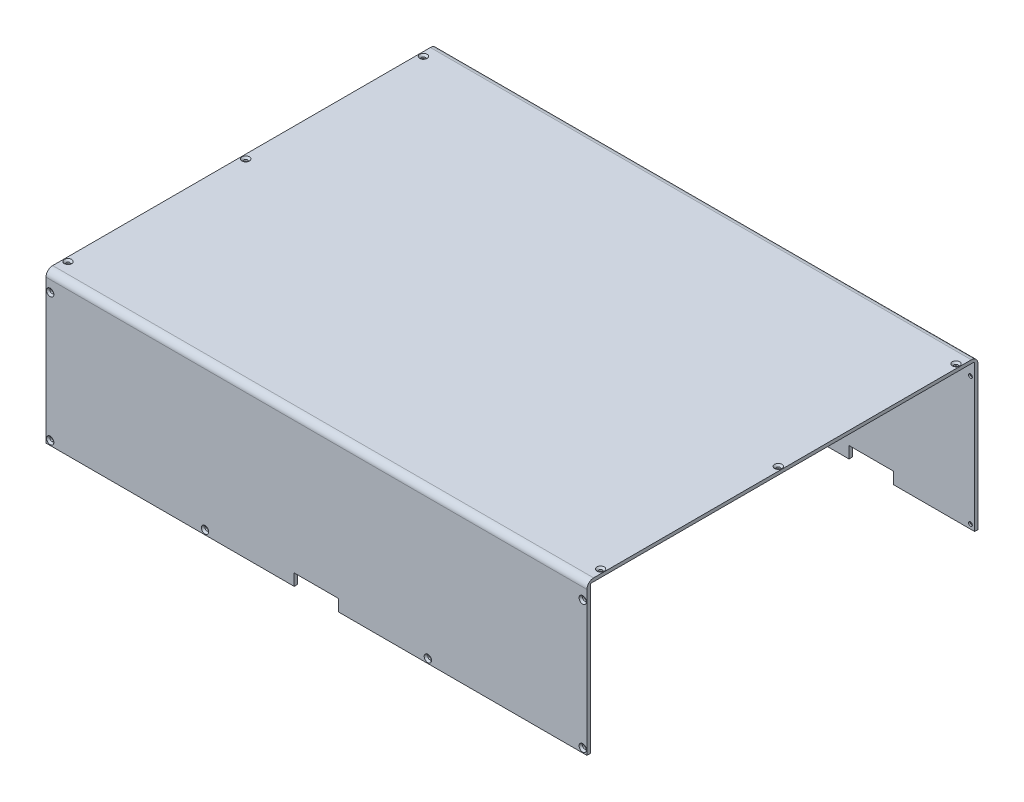
SolidWorks part; units mm, degrees
ref_plane "Front Plane" through (0, 0, 0) normal (0, 0, 1) x (1, 0, 0)
ref_plane "Top Plane" through (0, 0, 0) normal (0, 1, 0) x (1, 0, 0)
ref_plane "Right Plane" through (0, 0, 0) normal (1, 0, 0) x (0, 0, -1)
sketch "Sketch1" plane through (0, 0, 0) normal (0, 0, 1) x (1, 0, 0)
  line L1 (-242.75, 66) -> (242.75, 66)
  line L2 (-242.75, 66) -> (-242.75, -66)
  line L3 (-242.75, -66) -> (242.75, -66)
  line L4 (242.75, 66) -> (242.75, -66)
  line L5 (-242.75, 66) -> (242.75, -66) construction
  line L6 (-242.75, -66) -> (242.75, 66) construction
  point P0 (0, 0)
  dimension "D1" = 132
  dimension "D2" = 485.5
extrude "Boss-Extrude1" add sketch "Sketch1" along normal blind 3
sketch "Sketch2" plane through (0, 66, 0) normal (0, 1, 0) x (1, 0, 0)
  line L0 (-242.75, -3) -> (242.75, -3)
  line L1 (242.75, -3) -> (242.75, 348)
  line L2 (242.75, 348) -> (-242.75, 348)
  line L3 (-242.75, 348) -> (-242.75, -3)
  dimension "D1" = 351
extrude "Boss-Extrude2" add sketch "Sketch2" along normal blind 3
sketch "Sketch3" plane through (0, 66, 0) normal (0, -1, 0) x (1, 0, 0)
  line L0 (242.75, -348) -> (-242.75, -348)
  line L1 (-242.75, -348) -> (-242.75, -345)
  line L2 (-242.75, -348) -> (-242.75, 0) construction
  line L3 (-242.75, -345) -> (242.75, -345)
  line L4 (242.75, 0) -> (242.75, -348) construction
  line L5 (242.75, -345) -> (242.75, -348)
  dimension "D1" = 3
extrude "Boss-Extrude3" add sketch "Sketch3" along normal blind 132
fillet "Fillet1" radius 1 2 edges at (0, 66, -345) (0, 66, 0)
fillet "Fillet2" radius 6 2 edges at (0, 69, -348) (0, 69, 3)
sketch "Sketch4" plane through (0, 0, 3) normal (0, 0, 1) x (1, 0, 0)
  line L6 (20, -55.5) -> (20, -66) construction
  line L7 (-20, -55.5) -> (-20, -66) construction
  line L8 (20, -55.5) -> (20, -66)
  line L9 (-20, -55.5) -> (-20, -66)
  line L10 (-20, -66) -> (20, -66)
  line L11 (-20, -55.5) -> (20, -55.5)
extrude "Cut-Extrude1" cut sketch "Sketch4" against normal blind 4.5
sketch "Sketch5" plane through (0, 0, -348) normal (0, 0, -1) x (-1, 0, 0)
  line L12 (130, -66) -> (170, -66) construction
  line L13 (170, -66) -> (170, -55.5) construction
  line L14 (170, -55.5) -> (130, -55.5) construction
  line L15 (130, -55.5) -> (130, -66) construction
  line L16 (-170, -66) -> (-130, -66) construction
  line L17 (-130, -66) -> (-130, -55.5) construction
  line L18 (-130, -55.5) -> (-170, -55.5) construction
  line L19 (-170, -55.5) -> (-170, -66) construction
  line L20 (130, -66) -> (170, -66)
  line L21 (170, -66) -> (170, -55.5)
  line L22 (170, -55.5) -> (130, -55.5)
  line L23 (130, -55.5) -> (130, -66)
  line L24 (-170, -66) -> (-130, -66)
  line L25 (-130, -66) -> (-130, -55.5)
  line L26 (-130, -55.5) -> (-170, -55.5)
  line L27 (-170, -55.5) -> (-170, -66)
extrude "Cut-Extrude2" cut sketch "Sketch5" against normal blind 4.5
hole_wizard "Cross recess wood screw hole type 1" positions "Sketch6" profile "Sketch7" countersink size "M3" standard "GB" end condition through all
sketch "Sketch6" plane through (0, 69, 0) normal (0, 1, 0) x (1, 0, 0)
  point P0 (239, 332)
  point P3 (239, 172.5)
  point P6 (239, 13)
  point P9 (-239, 332)
  point P12 (-239, 172.5)
  point P15 (-239, 13)
sketch "Sketch7" plane through (239, 69, -332) normal (1, 0, 0) x (0, 0, 1)
  line L0 (0, 0) -> (0, 135)
  line L1 (0, 135) -> (1.7, 135)
  line L2 (1.7, 135) -> (1.7, 1.6)
  line L3 (1.7, 1.6) -> (3.3, 0)
  line L5 (3.3, 0) -> (0, 0)
  line L6 (-1.7, 1.6) -> (-3.3, 0) construction
  line L11 (0, -6.35) -> (0, 107.95) construction
  dimension "通孔孔直径" = 3.4
  dimension "通孔孔深度" = 135
  dimension "近端锥形沉头孔直径" = 6.6
  dimension "近端锥形沉头孔角度" = 90
hole_wizard "Cross recess wood screw hole type 2" positions "Sketch8" profile "Sketch10" countersink size "M3" standard "GB"
sketch "Sketch8" plane through (0, 0, 3) normal (0, 0, 1) x (1, 0, 0)
  point P0 (-239, 53)
  point P4 (-239, -62)
  point P7 (-100, -62)
  point P10 (100, -62)
  point P14 (239, 53)
  point P17 (239, -62)
sketch "Sketch10" plane through (-239, 53, 3) normal (1, 0, 0) x (0, -1, 0)
  line L0 (0, 0) -> (0, 7.5215)
  line L1 (0, 7.5215) -> (1.7, 6.5)
  line L2 (1.7, 6.5) -> (1.7, 1.6)
  line L3 (1.7, 1.6) -> (3.3, 0)
  line L5 (3.3, 0) -> (0, 0)
  line L6 (-1.7, 1.6) -> (-3.3, 0) construction
  line L10 (0, 7.5215) -> (-1.7, 6.5) construction
  line L11 (0, -6.35) -> (0, 107.95) construction
  dimension "孔直径" = 3.4
  dimension "孔深度" = 6.5
  dimension "近端锥形沉头孔直径" = 6.6
  dimension "近端锥形沉头孔角度" = 90
  dimension "导头角度" = 118
hole_wizard "Cross recess wood screw hole type 3" positions "Sketch11" profile "Sketch12" countersink size "M3" standard "GB"
sketch "Sketch11" plane through (0, 0, -348) normal (0, 0, -1) x (-1, 0, 0)
  point P0 (239, 53)
  point P3 (239, -62)
  point P6 (100, -62)
  point P9 (-100, -62)
  point P12 (-239, -62)
  point P15 (-239, 53)
sketch "Sketch12" plane through (-239, 53, -348) normal (1, 0, 0) x (0, 1, 0)
  line L0 (0, 0) -> (0, 7.5215)
  line L1 (0, 7.5215) -> (1.7, 6.5)
  line L2 (1.7, 6.5) -> (1.7, 1.6)
  line L3 (1.7, 1.6) -> (3.3, 0)
  line L5 (3.3, 0) -> (0, 0)
  line L6 (-1.7, 1.6) -> (-3.3, 0) construction
  line L10 (0, 7.5215) -> (-1.7, 6.5) construction
  line L11 (0, -6.35) -> (0, 107.95) construction
  dimension "孔直径" = 3.4
  dimension "孔深度" = 6.5
  dimension "近端锥形沉头孔直径" = 6.6
  dimension "近端锥形沉头孔角度" = 90
  dimension "导头角度" = 118
